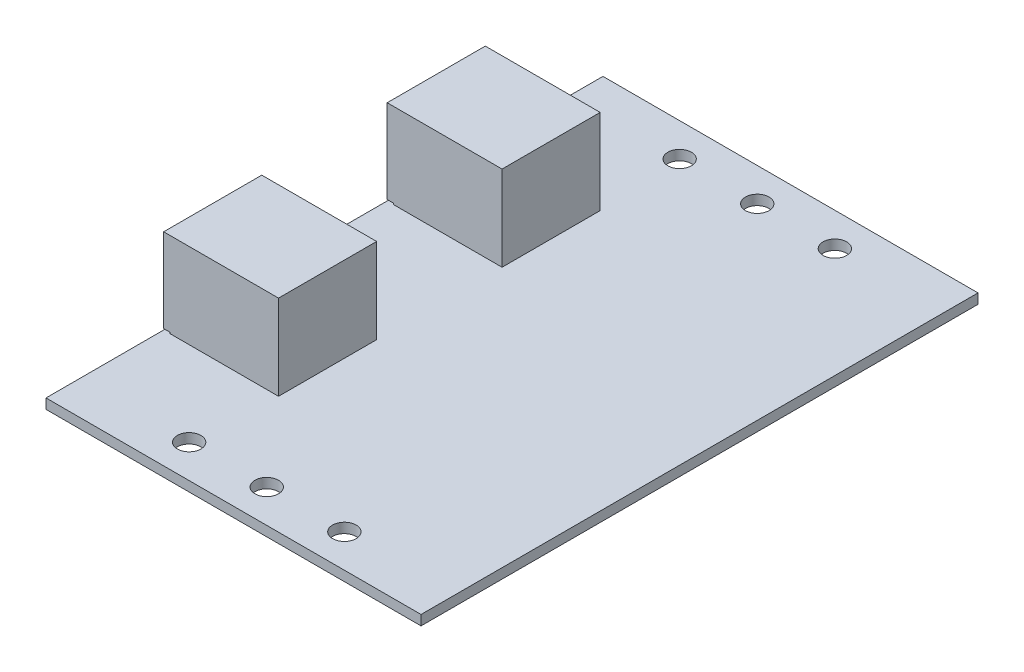
SolidWorks part; units mm, degrees
ref_plane "前视基准面" through (0, 0, 0) normal (0, 0, 1) x (1, 0, 0)
ref_plane "上视基准面" through (0, 0, 0) normal (0, 1, 0) x (1, 0, 0)
ref_plane "右视基准面" through (0, 0, 0) normal (1, 0, 0) x (0, 0, -1)
sketch "草图1" plane through (0, 0, 0) normal (0, 1, 0) x (1, 0, 0)
  line L1 (-30.2, 44.85) -> (30.2, 44.85)
  line L2 (-30.2, 44.85) -> (-30.2, -44.85)
  line L3 (-30.2, -44.85) -> (30.2, -44.85)
  line L4 (30.2, 44.85) -> (30.2, -44.85)
  line L5 (-30.2, 44.85) -> (30.2, -44.85) construction
  line L6 (-30.2, -44.85) -> (30.2, 44.85) construction
  point P0 (0, 0)
  dimension "D1" = 60.4
  dimension "D2" = 89.7
extrude "凸台-拉伸1" add sketch "草图1" along normal blind 1.6
sketch "草图2" plane through (0, 1.6, 0) normal (0, 1, 0) x (1, 0, 0)
  line L1 (-12.5, 39.5) -> (12.5, 39.5) construction
  line L2 (-12.5, 39.5) -> (-12.5, -39.5) construction
  line L3 (-12.5, -39.5) -> (12.5, -39.5) construction
  line L4 (12.5, 39.5) -> (12.5, -39.5) construction
  line L5 (-12.5, 39.5) -> (12.5, -39.5) construction
  line L6 (-12.5, -39.5) -> (12.5, 39.5) construction
  circle A0 centre (-12.5, -39.5) radius 1.9
  circle A1 centre (12.5, -39.5) radius 1.9
  circle A2 centre (-12.5, 39.5) radius 1.9
  circle A3 centre (12.5, 39.5) radius 1.9
  circle A4 centre (0, 39.5) radius 1.9
  circle A5 centre (0, -39.5) radius 1.9
  point P0 (0, 0)
  dimension "D1" = 3.8
  dimension "D2" = 25
  dimension "D3" = 79
extrude "切除-拉伸1" cut sketch "草图2" against normal blind 1.6
sketch "草图3" plane through (-30.2, 0, 0) normal (-1, 0, 0) x (0, 0, 1)
  line L0 (0, 0) -> (0, 13.8824) construction
  line L1 (10.1, 15.3) -> (25.9, 15.3)
  line L2 (10.1, 15.3) -> (10.1, 1.6)
  line L3 (10.1, 1.6) -> (25.9, 1.6)
  line L4 (25.9, 15.3) -> (25.9, 1.6)
  line L5 (-25.9, 15.3) -> (-10.1, 15.3)
  line L6 (-25.9, 15.3) -> (-25.9, 1.6)
  line L7 (-25.9, 1.6) -> (-10.1, 1.6)
  line L8 (-10.1, 15.3) -> (-10.1, 1.6)
  line L9 (-44.85, 1.6) -> (44.85, 1.6) construction
  line L10 (-44.85, 0) -> (44.85, 0) construction
  dimension "D1" = 15.8
  dimension "D2" = 15.3
  dimension "D3" = 36
extrude "凸台-拉伸2" add sketch "草图3" against normal blind 18.5
sketch "草图4" plane through (-30.2, 0, 0) normal (-1, 0, 0) x (0, 0, 1)
  line L0 (25.9, 1.6) -> (25.9, 15.3) construction
  line L1 (-25.9, 1.6) -> (25.9, 1.6)
  line L2 (-25.9, 1.6) -> (-25.9, 1.8)
  line L3 (-25.9, 1.8) -> (25.9, 1.8)
  line L4 (25.9, 1.6) -> (25.9, 1.8)
  dimension "D1" = 0.2
extrude "切除-拉伸2" cut sketch "草图4" against normal blind 1
